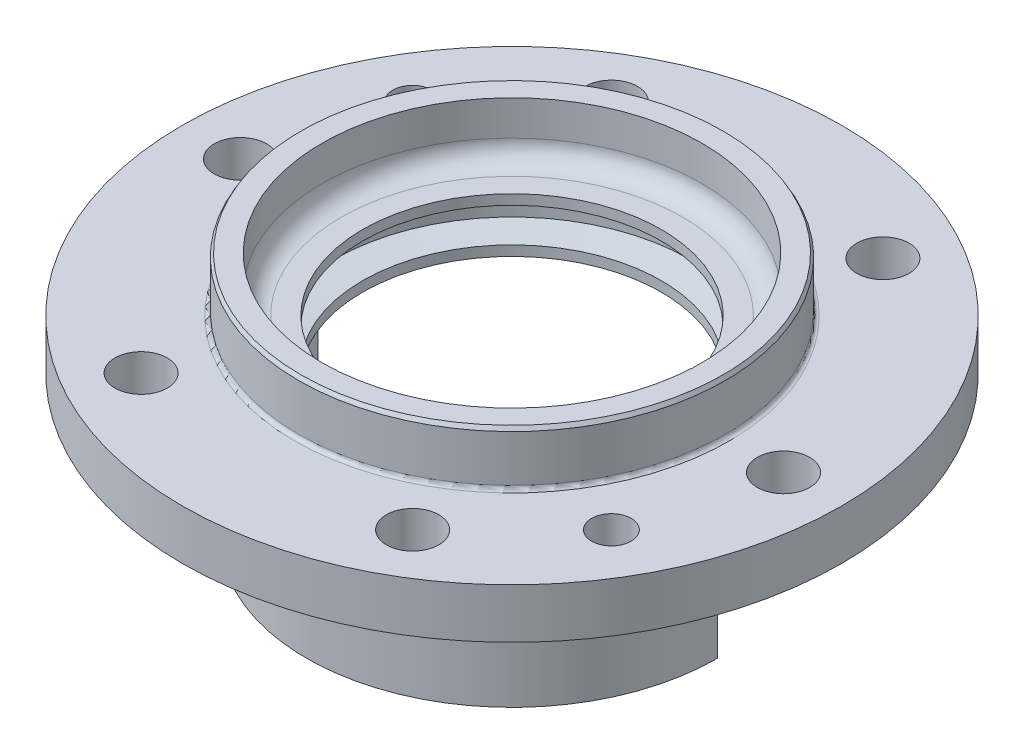
SolidWorks part; units mm, degrees
ref_plane "Front Plane" through (0, 0, 0) normal (0, 0, 1) x (1, 0, 0)
ref_plane "Top Plane" through (0, 0, 0) normal (0, 1, 0) x (1, 0, 0)
ref_plane "Right Plane" through (0, 0, 0) normal (1, 0, 0) x (0, 0, -1)
sketch "Sketch1" plane through (0, 0, 0) normal (0, 1, 0) x (1, 0, 0)
  circle A0 centre (0, 0) radius 85
  dimension "D1" = 170
extrude "Boss-Extrude1" add sketch "Sketch1" along normal blind 14
sketch "Sketch2" plane through (0, 14, 0) normal (0, 1, 0) x (1, 0, 0)
  circle A0 centre (0, 0) radius 55
  circle A1 centre (0, 0) radius 49
  dimension "D1" = 98
  dimension "D2" = 110
extrude "Boss-Extrude2" add sketch "Sketch2" along normal blind 14
fillet "Fillet1" radius 5 1 edges at (0, 14, 49)
fillet "Fillet2" radius 1 1 edges at (0, 14, 55)
chamfer "Chamfer1" distance 2 angle 30 1 edges at (0, 0, 85)
chamfer "Chamfer2" distance 1 angle 30 1 edges at (0, 28, 55)
sketch "Sketch3" plane through (0, 0, 0) normal (0, -1, 0) x (1, 0, 0)
  line L0 (-53, 0) -> (-50, 0)
  line L1 (50, 0) -> (53, 0)
  arc A0 (50, 0) -> (-50, 0) centre (0, 0) ccw
  arc A2 (53, 0) -> (-53, 0) centre (0, 0) ccw
  circle A4 centre (0, 0) radius 53 construction
  circle A5 centre (0, 0) radius 50 construction
  point P3 (53, 0)
  point P8 (0, 0)
  point P13 (47.8152, 14.6186)
  dimension "D1" = 100
  dimension "D2" = 3
extrude "Boss-Extrude3" add sketch "Sketch3" along normal blind 36
sketch "Sketch4" plane through (0, 0, 0) normal (0, 0, 1) x (1, 0, 0)
  line L0 (0, 0) -> (0, 14) construction
  line L1 (85, 14) -> (-85, 14) construction
  line L2 (0, 7) -> (-96.0902, 7) construction
  line L3 (-46, 10.5) -> (-46, 3.5)
  line L4 (-46, 10.5) -> (-38.5, 11.4209)
  line L5 (-46, 3.5) -> (-38.5, 2.5791)
  line L6 (-38.5, 11.4209) -> (-38.5, 14)
  line L7 (-38.5, 2.5791) -> (-38.5, 0)
  line L13 (0, 14) -> (-38.5, 14)
  line L14 (0, 0) -> (-38.5, 0)
  line L15 (0, 14) -> (0, 0)
  line L16 (-53, 0) -> (53, 0) construction
  line L17 (44, 14) -> (-44, 14) construction
  point P10 (-46, 7)
  dimension "D1" = 7
  dimension "D2" = 46
  dimension "D3" = 14
  dimension "D4" = 38.5
revolve "Cut-Revolve1" cut sketch "Sketch4" angle 360 about L15
sketch "Sketch5" plane through (0, 0, 0) normal (0, -1, 0) x (1, 0, 0)
  line L0 (0, 0) -> (0, 100.6637) construction
  line L1 (0, 0) -> (-35, 60.6218) construction
  circle A0 centre (-35, 60.6218) radius 6.75
  dimension "D3" = 13.5
  dimension "D1" = 30
  dimension "D2" = 70
extrude "Cut-Extrude1" cut sketch "Sketch5" against normal through all
pattern_circular "CirPattern1" count 6 over 360 about axis through (0, 0, 0) along (0, 1, 0) of "Cut-Extrude1"
sketch "Sketch6" plane through (0, 0, 0) normal (0, -1, 0) x (1, 0, 0)
  line L0 (0, 0) -> (-70, 0) construction
  line L1 (0, 0) -> (-60.6218, -35) construction
  line L2 (0, 0) -> (60.6218, 35) construction
  dimension "D1" = 70
  dimension "D2" = 30
hole_wizard "M12 Tapped Hole1" positions "Sketch7" profile "Sketch8" tap size "M12" standard "GB" end condition through all
sketch "Sketch7" plane through (0, 0, 0) normal (0, -1, 0) x (-1, 0, 0)
  point P0 (-60.6218, -35)
  point P3 (60.6218, 35)
sketch "Sketch8" plane through (60.6218, 0, 35) normal (1, 0, 0) x (0, 0, -1)
  line L0 (0, 0) -> (0, 28)
  line L1 (0, 28) -> (5.1, 28)
  line L2 (5.1, 28) -> (5.1, 0)
  line L5 (5.1, 0) -> (0, 0)
  line L11 (0, -6.35) -> (0, 107.95) construction
  dimension "通孔螺纹孔钻头直径" = 10.2
  dimension "通孔螺纹孔钻头深度" = 28
cosmetic thread "Cosmetic Thread1" parameters "D2"=12
cosmetic thread "Cosmetic Thread2" parameters "D2"=12
